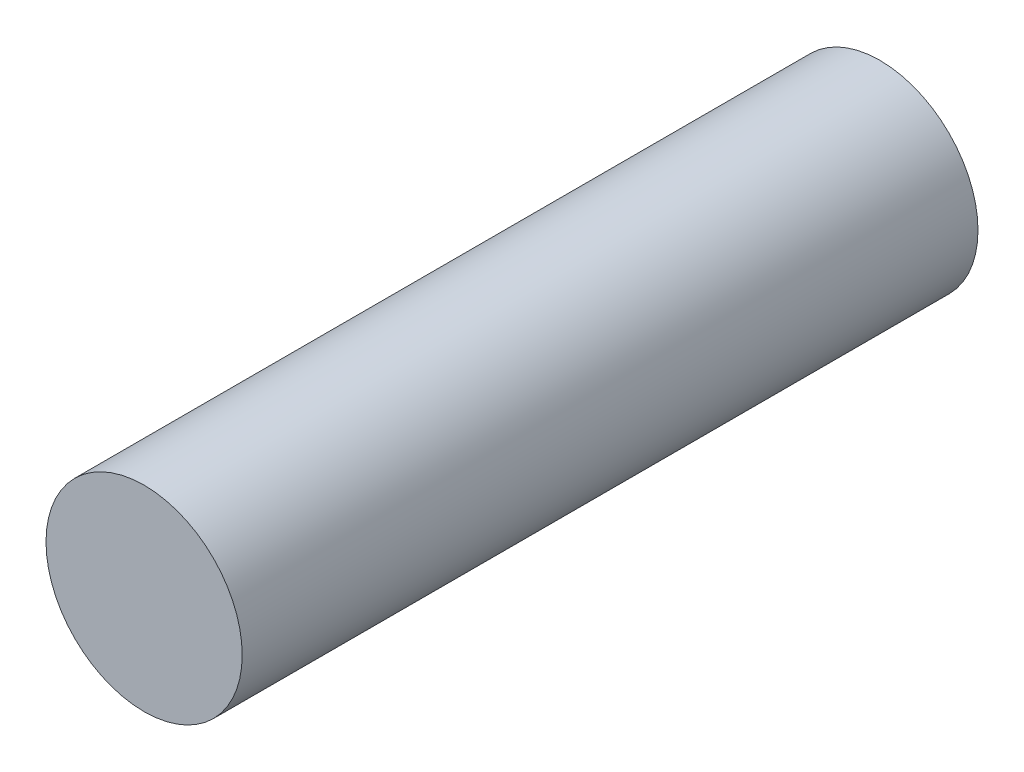
from build123d import *

# Parameters (mm, degrees)
SKETCH1_R           = 12
BOSS_EXTRUDE1_DEPTH = 90


with BuildPart() as part:
    # Sketch1 → Boss-Extrude1 (new body)
    with BuildSketch(Plane.XY):
        with Locations(Location((0, 0, 0), (0, 0, 180))):
            Circle(SKETCH1_R)
    extrude(amount=BOSS_EXTRUDE1_DEPTH)


solid = part.part
